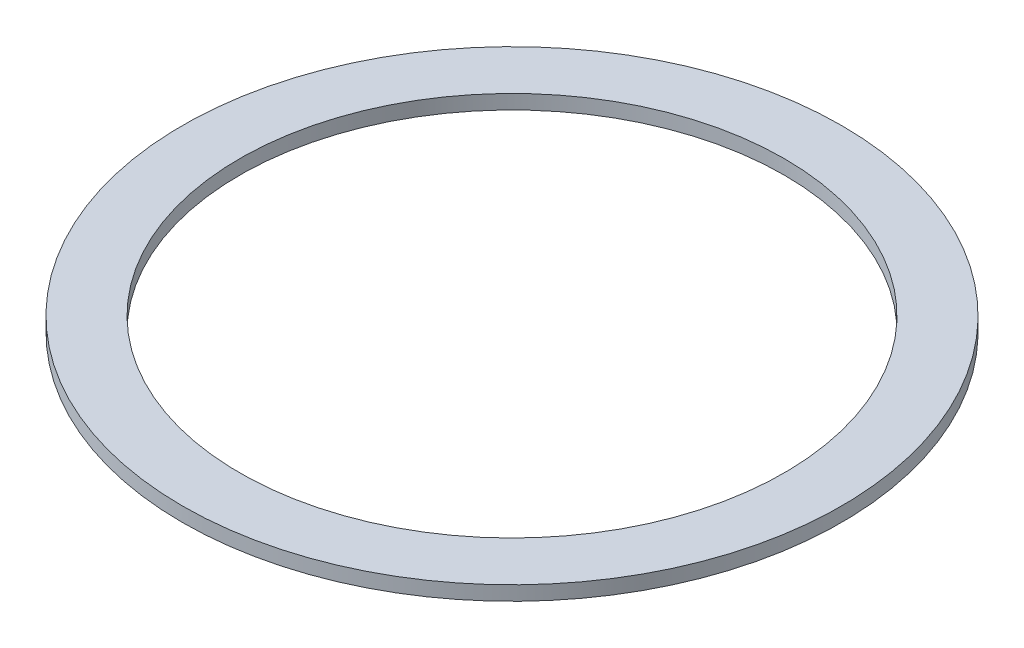
SolidWorks part; units mm, degrees
ref_plane "Front" through (0, 0, 0) normal (0, 0, 1) x (1, 0, 0)
ref_plane "Top" through (0, 0, 0) normal (0, 1, 0) x (1, 0, 0)
ref_plane "Right" through (0, 0, 0) normal (1, 0, 0) x (0, 0, -1)
sketch "Sketch1" plane through (0, 0, 0) normal (0, 0, 1) x (1, 0, 0)
  line L0 (0, 0) -> (0, 27.2) construction
  line L1 (19, 0) -> (23, 0)
  line L2 (19, 0) -> (19, 1)
  line L3 (19, 1) -> (23, 1)
  line L4 (23, 0) -> (23, 1)
  dimension "D1" = 1
  dimension "D2" = 4
  dimension "D3" = 19
revolve "Revolve1" add sketch "Sketch1" angle 360 about L0
